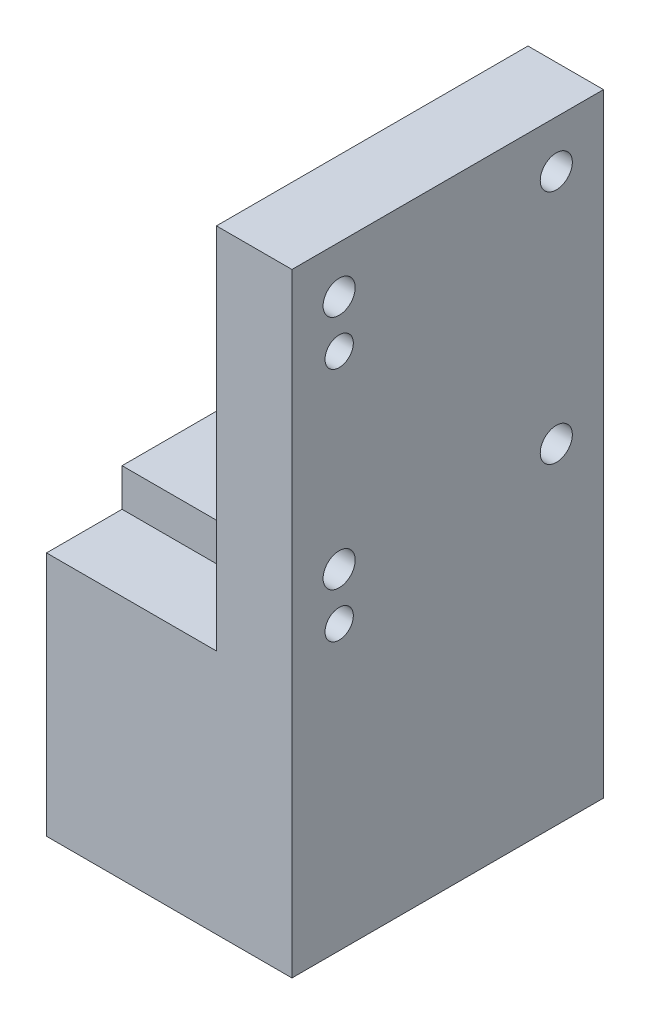
from build123d import *

# Parameters (mm, degrees)
SKETCH_1_W                                        = 33
SKETCH_1_H                                        = 65
BOSS_EXTRUDE_1_DEPTH                              = 8
SKETCH_2_W                                        = 33
SKETCH_2_H                                        = 30
BOSS_EXTRUDE_2_DEPTH                              = 18
M3_HEX_SOCKET_CAP_SCREW_COUNTERBORE_1_D           = 3.4
M3_HEX_SOCKET_CAP_SCREW_COUNTERBORE_1_CBORE_D     = 6.5
M3_HEX_SOCKET_CAP_SCREW_COUNTERBORE_1_CBORE_DEPTH = 3
LINEAR_PATTERN_1_COUNT                            = 2
LINEAR_PATTERN_1_PITCH                            = 23
LINEAR_PATTERN_1_COUNT_DIR2                       = 2
LINEAR_PATTERN_1_PITCH_DIR2                       = 25
LINEAR_PATTERN_3_COUNT                            = 3
LINEAR_PATTERN_3_PITCH                            = 10
SKETCH_9_W                                        = 1.5
SKETCH_9_H                                        = 8
LINEAR_PATTERN_4_COUNT                            = 2
LINEAR_PATTERN_4_PITCH                            = 25
SKETCH_11_W                                       = 8
SKETCH_11_H                                       = 4
CUT_EXTRUDE_1_DEPTH                               = 18
LINEAR_PATTERN_5_COUNT                            = 2
LINEAR_PATTERN_5_PITCH                            = 20


with BuildPart() as part:
    # Sketch 1 → Boss-Extrude 1 (new body)
    with BuildSketch(Plane(origin=(0, 0, 0), x_dir=(0, 0, -1), z_dir=(1, 0, 0))):
        Rectangle(SKETCH_1_W, SKETCH_1_H)
    extrude(amount=BOSS_EXTRUDE_1_DEPTH)

    # Sketch 2 → Boss-Extrude 2 (add)
    with BuildSketch(Plane.ZY):
        with Locations((0, -17.5)):
            Rectangle(SKETCH_2_W, SKETCH_2_H)
    extrude(amount=BOSS_EXTRUDE_2_DEPTH)

    # M3 Hex Socket Cap Screw Counterbore 1 (through all)
    with Locations(Plane.ZY):
        with Locations((-11.5, 27.5)):
            m3_hex_socket_cap_screw_counterbore_1 = CounterBoreHole(M3_HEX_SOCKET_CAP_SCREW_COUNTERBORE_1_D / 2, M3_HEX_SOCKET_CAP_SCREW_COUNTERBORE_1_CBORE_D / 2, M3_HEX_SOCKET_CAP_SCREW_COUNTERBORE_1_CBORE_DEPTH)

    # Linear Pattern 1: M3 Hex Socket Cap Screw Counterbore 1 2 × 2
    with Locations(*[(0, -j * LINEAR_PATTERN_1_PITCH_DIR2, i * LINEAR_PATTERN_1_PITCH) for i in range(LINEAR_PATTERN_1_COUNT) for j in range(LINEAR_PATTERN_1_COUNT_DIR2) if (i, j) != (0, 0)]):
        add(m3_hex_socket_cap_screw_counterbore_1, mode=Mode.SUBTRACT)

    # Sketch 7 → M4 Tapped Hole 2 (revolve, cut)
    with BuildSketch(Plane(origin=(-18, -27.5, 0), x_dir=(0, 0, 1), z_dir=(0, 1, 0))):
        Polygon((0, 0), (0, 11.091420021), (1.65, 10.1), (1.65, 0), align=None)
    m4_tapped_hole_2 = revolve(axis=Axis((-24.35, -27.5, 0), (1, 0, 0)), mode=Mode.SUBTRACT)

    # Linear Pattern 3: M4 Tapped Hole 2 ×3
    with Locations(*[(0, i * LINEAR_PATTERN_3_PITCH, 0) for i in range(1, LINEAR_PATTERN_3_COUNT)]):
        add(m4_tapped_hole_2, mode=Mode.SUBTRACT)

    # Sketch 9 → Ø3.0 (3) Hole 1 (revolve, cut)
    with BuildSketch(Plane(origin=(0, 22.5, 11.5), x_dir=(0, 0, 1), z_dir=(0, 1, 0))):
        with Locations((0.75, 4)):
            Rectangle(SKETCH_9_W, SKETCH_9_H)
    f_3_0_3_hole_1 = revolve(axis=Axis((-6.35, 22.5, 11.5), (1, 0, 0)), mode=Mode.SUBTRACT)

    # Linear Pattern 4: Ø3.0 (3) Hole 1 ×2
    with Locations(*[(0, -i * LINEAR_PATTERN_4_PITCH, 0) for i in range(1, LINEAR_PATTERN_4_COUNT)]):
        add(f_3_0_3_hole_1, mode=Mode.SUBTRACT)

    # Sketch 11 → Cut-Extrude 1 (cut)
    with BuildSketch(Plane.ZY.offset(18)):
        with Locations((12.5, -4.5)):
            Rectangle(SKETCH_11_W, SKETCH_11_H)
    extrude(amount=-CUT_EXTRUDE_1_DEPTH, mode=Mode.SUBTRACT)

    # Sketch 12 → Ø4.0 (4) Hole 1 (revolve, cut)
    with BuildSketch(Plane(origin=(-18, -10, -10), x_dir=(0, 0, 1), z_dir=(0, 1, 0))):
        Polygon((0, 0), (0, 11.201721238), (2, 10), (2, 0), align=None)
    f_4_0_4_hole_1 = revolve(axis=Axis((-24.35, -10, -10), (1, 0, 0)), mode=Mode.SUBTRACT)

    # Linear Pattern 5: Ø4.0 (4) Hole 1 ×2
    with Locations(*[(0, 0, i * LINEAR_PATTERN_5_PITCH) for i in range(1, LINEAR_PATTERN_5_COUNT)]):
        add(f_4_0_4_hole_1, mode=Mode.SUBTRACT)


solid = part.part
